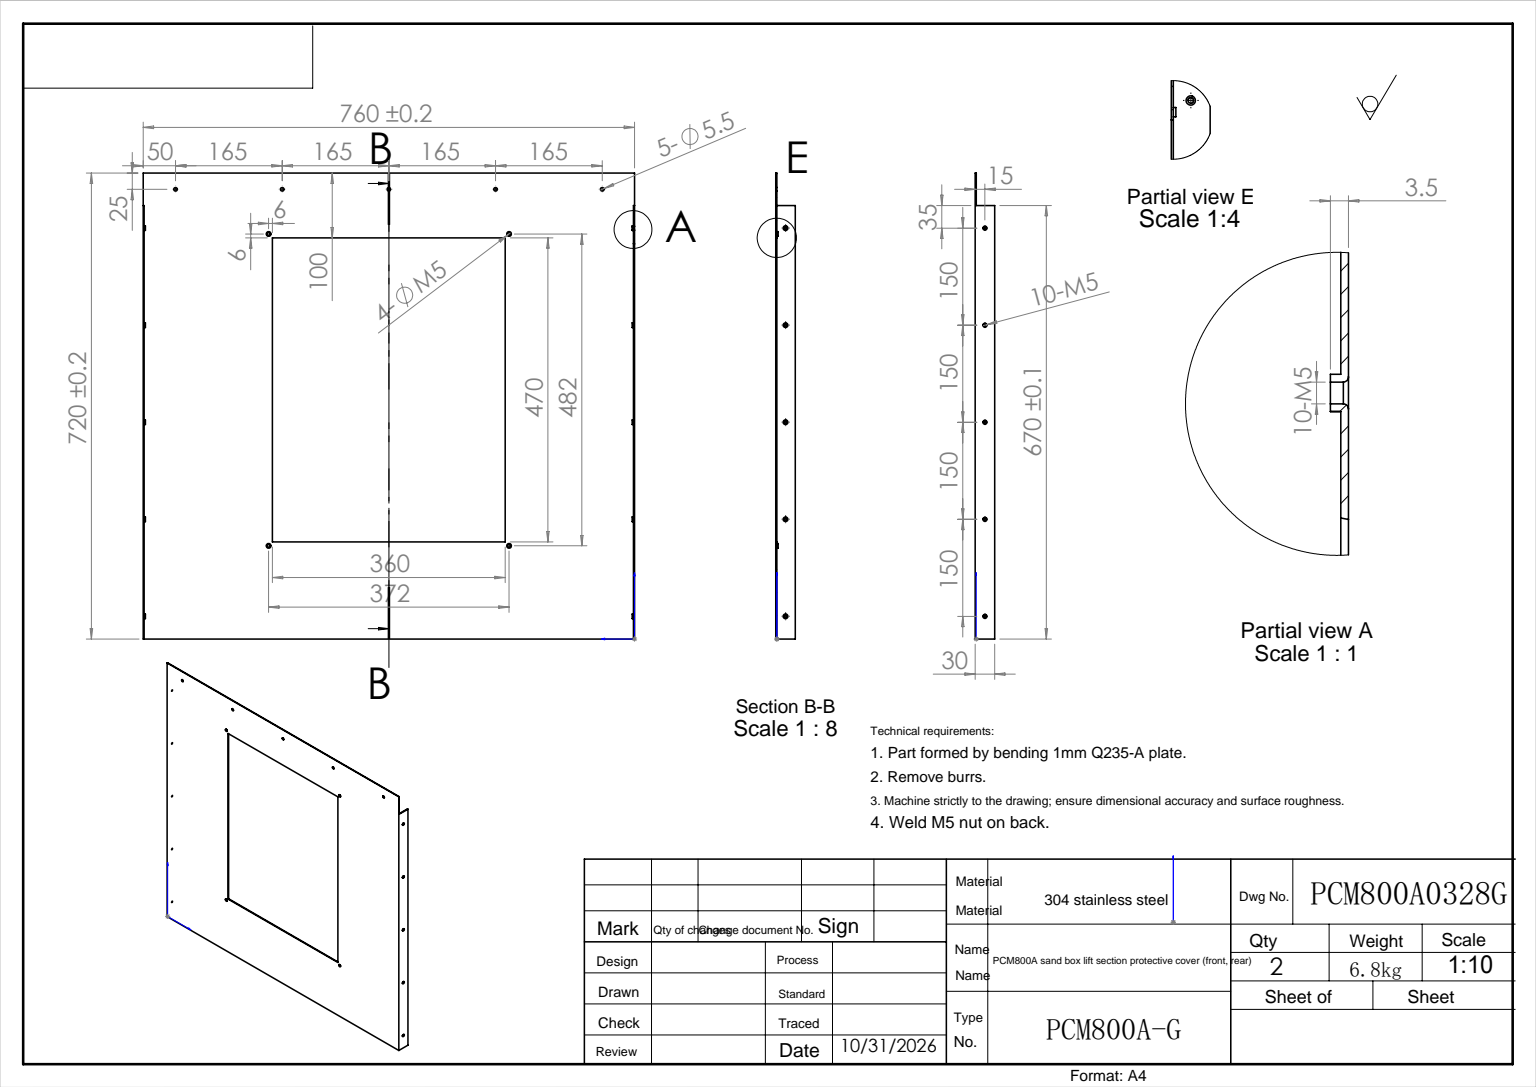
SolidWorks part; units mm, degrees
ref_plane "前视基准面" through (0, 0, 0) normal (0, 0, 1) x (1, 0, 0)
ref_plane "上视基准面" through (0, 0, 0) normal (0, 1, 0) x (1, 0, 0)
ref_plane "右视基准面" through (0, 0, 0) normal (1, 0, 0) x (0, 0, -1)
sketch "草图1" plane through (0, 0, 0) normal (0, 0, 1) x (1, 0, 0)
  line L1 (0, 0) -> (760, 0)
  line L2 (0, 0) -> (0, 720)
  line L3 (0, 720) -> (760, 720)
  line L4 (760, 0) -> (760, 720)
  dimension "D1" = 760
  dimension "D2" = 720
extrude "凸台-拉伸1" add sketch "草图1" along normal blind 1.5
sketch "草图2" plane through (0, 0, 0) normal (0, 0, -1) x (-1, 0, 0)
  line L0 (-760, 720) -> (0, 720) construction
  line L1 (-760, 0) -> (-758.5, 0)
  line L2 (-760, 0) -> (-760, 670)
  line L3 (-760, 670) -> (-758.5, 670)
  line L4 (-758.5, 0) -> (-758.5, 670)
  line L5 (0, 0) -> (-1.5, 0)
  line L6 (0, 0) -> (0, 670)
  line L7 (0, 670) -> (-1.5, 670)
  line L8 (-1.5, 0) -> (-1.5, 670)
  dimension "D1" = 1.5
  dimension "D2" = 1.5
  dimension "D3" = 50
  dimension "D4" = 50
extrude "凸台-拉伸2" add sketch "草图2" along normal blind 28.5
sketch "草图3" plane through (0, 0, 0) normal (0, 0, -1) x (-1, 0, 0)
  line L0 (-760, 670) -> (-760, 720) construction
  line L1 (-760, 720) -> (0, 720) construction
  circle A0 centre (-710, 695) radius 2.75
  circle A1 centre (-545, 695) radius 2.75
  circle A2 centre (-380, 695) radius 2.75
  circle A3 centre (-215, 695) radius 2.75
  circle A4 centre (-50, 695) radius 2.75
  dimension "D1" = 5.5
  dimension "D2" = 50
  dimension "D3" = 25
  dimension "D4" = 5
extrude "切除-拉伸1" cut sketch "草图3" against normal blind 30
sketch "草图5" plane through (1.5, 0, 0) normal (1, 0, 0) x (0, 0, -1)
  line L1 (28.5, 670) -> (0, 670) construction
  line L2 (28.5, 670) -> (28.5, 0) construction
  circle A0 centre (13.5, 635) radius 3.6
  circle A1 centre (13.5, 485) radius 3.6
  circle A2 centre (13.5, 335) radius 3.6
  circle A3 centre (13.5, 185) radius 3.6
  circle A4 centre (13.5, 35) radius 3.6
  dimension "D1" = 7.2
  dimension "D2" = 35
  dimension "D3" = 15
  dimension "D4" = 5
extrude "凸台-拉伸3" add sketch "草图5" along normal blind 2
sketch "草图6" plane through (758.5, 0, 0) normal (-1, 0, 0) x (0, 0, 1)
  circle A2 centre (-13.5, 635) radius 3.6
  circle A3 centre (-13.5, 635) radius 3.6
  circle A5 centre (-13.5, 485) radius 3.6
  circle A6 centre (-13.5, 485) radius 3.6
  circle A8 centre (-13.5, 335) radius 3.6
  circle A9 centre (-13.5, 335) radius 3.6
  circle A11 centre (-13.5, 185) radius 3.6
  circle A12 centre (-13.5, 185) radius 3.6
  circle A14 centre (-13.5, 35) radius 3.6
  circle A15 centre (-13.5, 35) radius 3.6
  dimension "D1" = 0
  dimension "D2" = 0
  dimension "D3" = 0
  dimension "D4" = 0
  dimension "D5" = 0
extrude "凸台-拉伸4" add sketch "草图6" along normal blind 2
hole_wizard "M5 螺纹孔1" positions "草图8" profile "草图7" tap size "M5" standard "GB" end condition through all
sketch "草图8" plane through (0, 0, 0) normal (-1, 0, 0) x (0, 0, 1)
  point P0 (-13.5, 635)
  point P1 (-13.5, 485)
  point P4 (-13.5, 335)
  point P7 (-13.5, 185)
  point P10 (-13.5, 35)
sketch "草图7" plane through (0, 635, -13.5) normal (0, 1, 0) x (0, 0, 1)
  line L0 (0, 0) -> (0, 760)
  line L1 (0, 760) -> (2.1, 760)
  line L2 (2.1, 760) -> (2.1, 0)
  line L5 (2.1, 0) -> (0, 0)
  line L11 (0, -6.35) -> (0, 107.95) construction
  dimension "通孔螺纹孔钻头直径" = 4.2
  dimension "通孔螺纹孔钻头深度" = 760
cosmetic thread "孔螺蚊线1" parameters "D2"=5
cosmetic thread "孔螺蚊线2" parameters "D2"=5
cosmetic thread "孔螺蚊线3" parameters "D2"=5
cosmetic thread "孔螺蚊线4" parameters "D2"=5
cosmetic thread "孔螺蚊线5" parameters "D2"=5
fillet "圆角2" radius 1 10 edges at (760, 35, -11.4) (760, 185, -11.4) (760, 335, -11.4) (760, 485, -11.4) (760, 635, -11.4) (0, 35, -11.4) (0, 185, -11.4) (0, 335, -11.4) (0, 485, -11.4) (0, 635, -11.4)
sketch "草图9" plane through (0, 0, 1.5) normal (0, 0, 1) x (1, 0, 0)
  line L0 (0, 720) -> (0, 0) construction
  line L1 (200, 620) -> (560, 620)
  line L2 (200, 620) -> (200, 150)
  line L3 (200, 150) -> (560, 150)
  line L4 (560, 620) -> (560, 150)
  line L5 (760, 0) -> (760, 720) construction
  line L6 (760, 720) -> (0, 720) construction
  line L7 (0, 0) -> (760, 0) construction
  dimension "D1" = 200
  dimension "D2" = 200
  dimension "D3" = 100
  dimension "D4" = 150
extrude "切除-拉伸2" cut sketch "草图9" against normal blind 10
sketch "草图10" plane through (0, 0, 0) normal (0, 0, -1) x (-1, 0, 0)
  line L0 (-560, 620) -> (-560, 150) construction
  line L1 (-200, 150) -> (-200, 620) construction
  line L2 (-200, 620) -> (-560, 620) construction
  line L3 (-560, 150) -> (-200, 150) construction
  circle A0 centre (-566, 626) radius 3.6
  circle A1 centre (-194, 626) radius 3.6
  circle A2 centre (-194, 144) radius 3.6
  circle A3 centre (-566, 144) radius 3.6
  dimension "D1" = 7.2
  dimension "D2" = 7.2
  dimension "D3" = 7.2
  dimension "D4" = 7.2
  dimension "D9" = 6
  dimension "D11" = 6
  dimension "D12" = 6
  dimension "D5" = 6
  dimension "D6" = 6
  dimension "D7" = 6
  dimension "D8" = 6
  dimension "D10" = 6
extrude "凸台-拉伸5" add sketch "草图10" along normal blind 2
sketch "草图11" plane through (0, 0, -2) normal (0, 0, -1) x (-1, 0, 0)
  circle A0 centre (-566, 626) radius 2.1
  circle A1 centre (-194, 626) radius 2.1
  circle A2 centre (-194, 144) radius 2.1
  circle A3 centre (-566, 144) radius 2.1
  dimension "D1" = 4.2
  dimension "D2" = 4.2
  dimension "D3" = 4.2
  dimension "D4" = 4.2
extrude "切除-拉伸3" cut sketch "草图11" against normal blind 112
fillet "圆角3" radius 1 4 edges at (563.9, 626, 1.5) (191.9, 626, 1.5) (191.9, 144, 1.5) (563.9, 144, 1.5)
